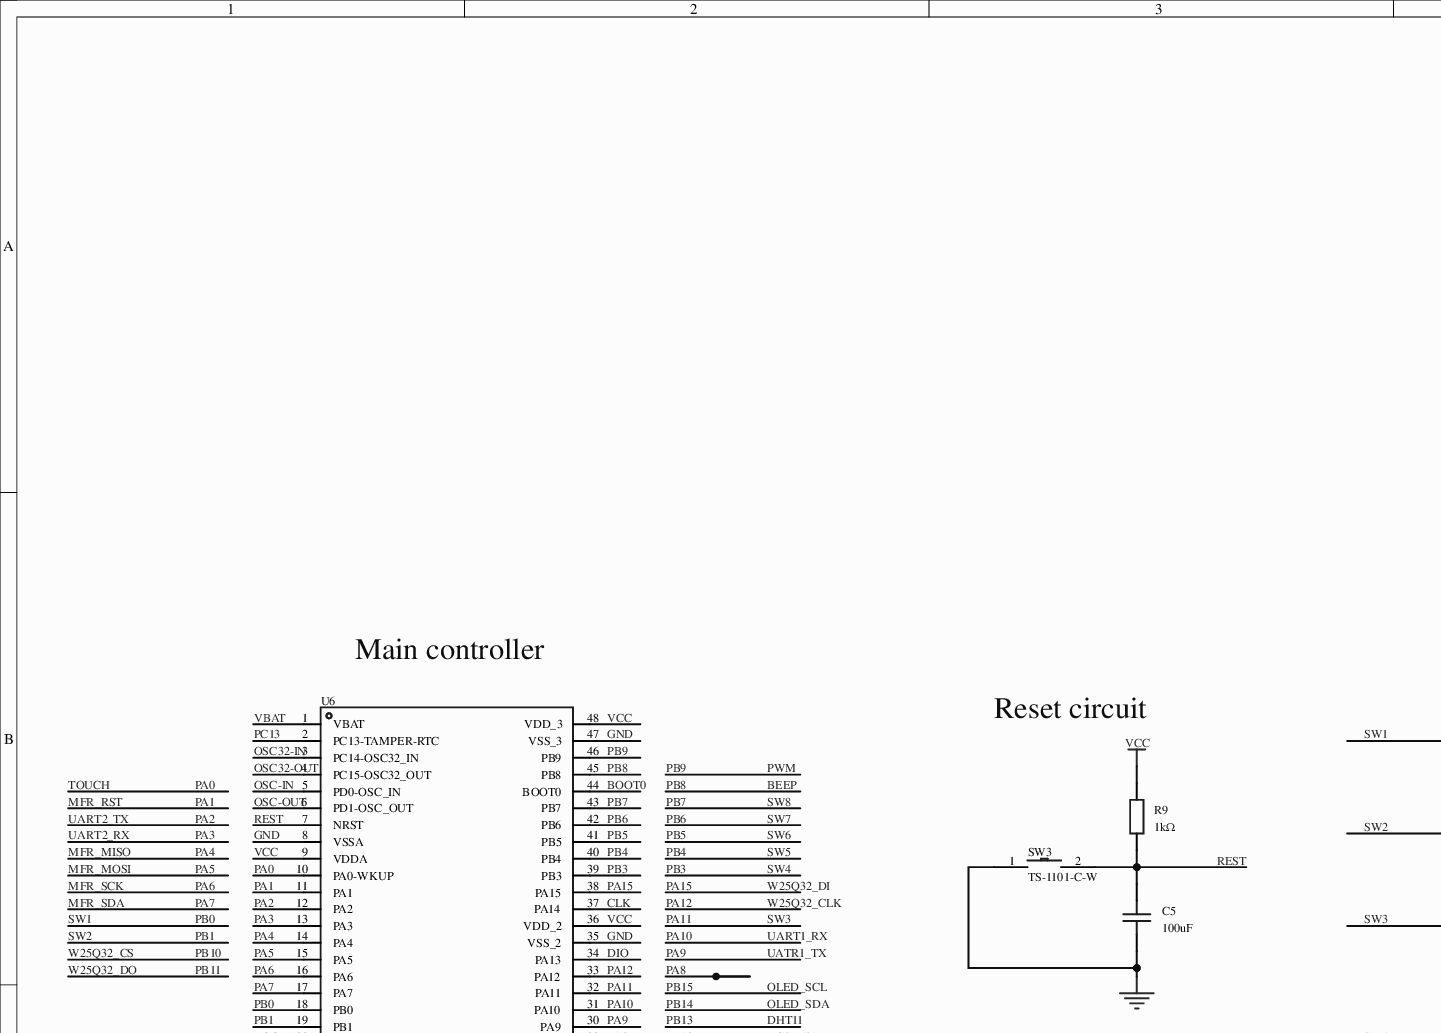
[diagram p0: MISC51820-3.schdoc, top left]
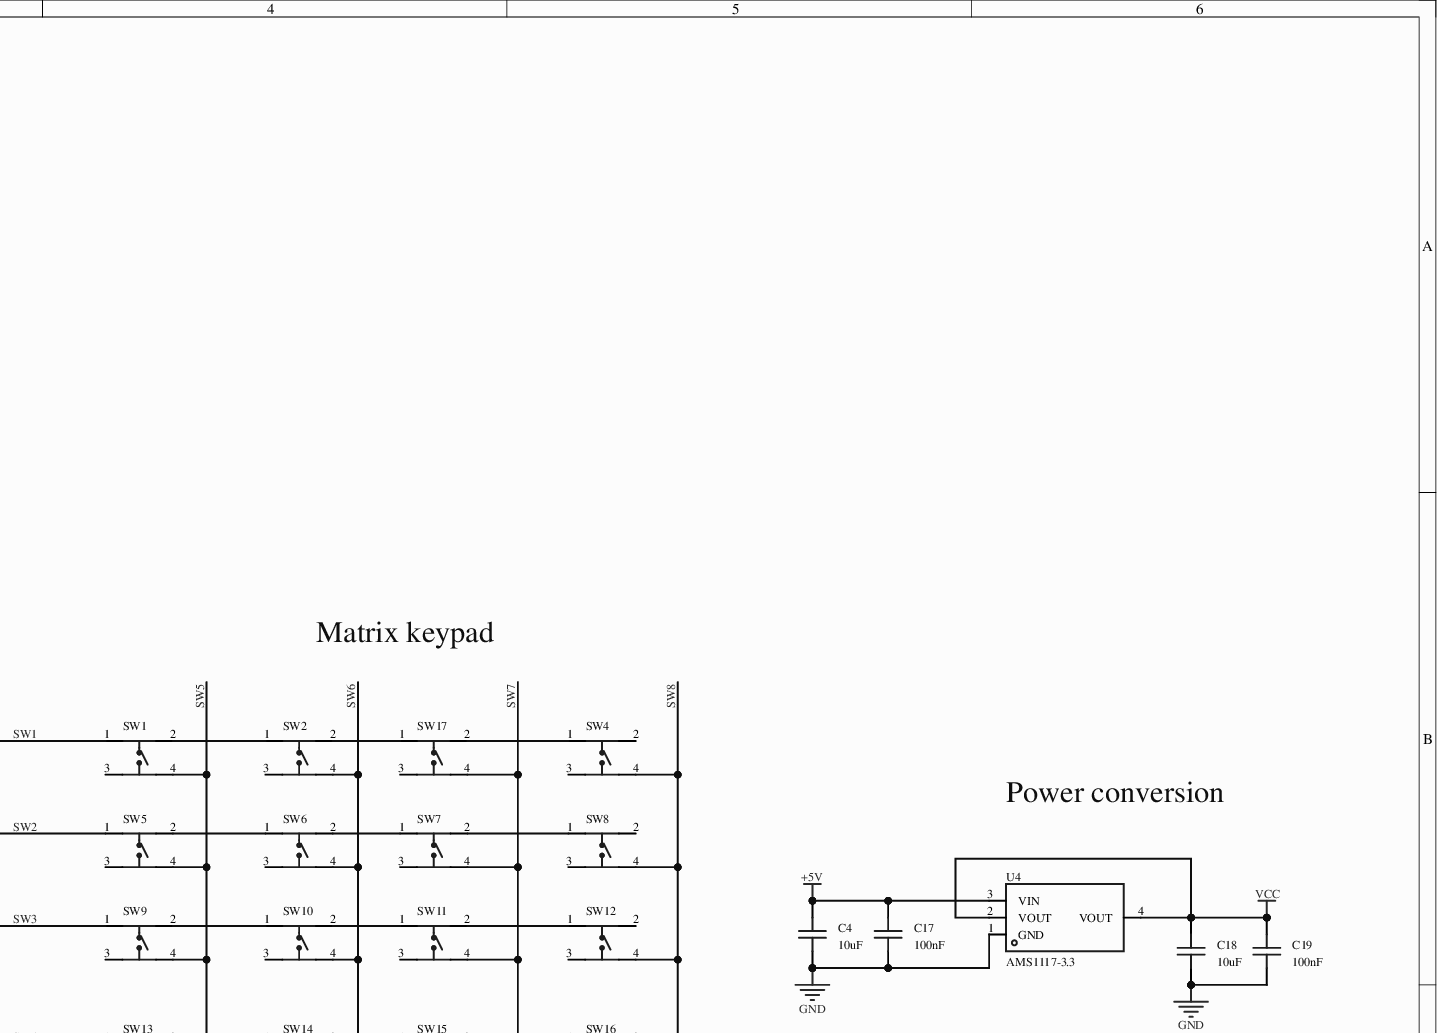
[diagram p1: MISC51820-3.schdoc, top right]
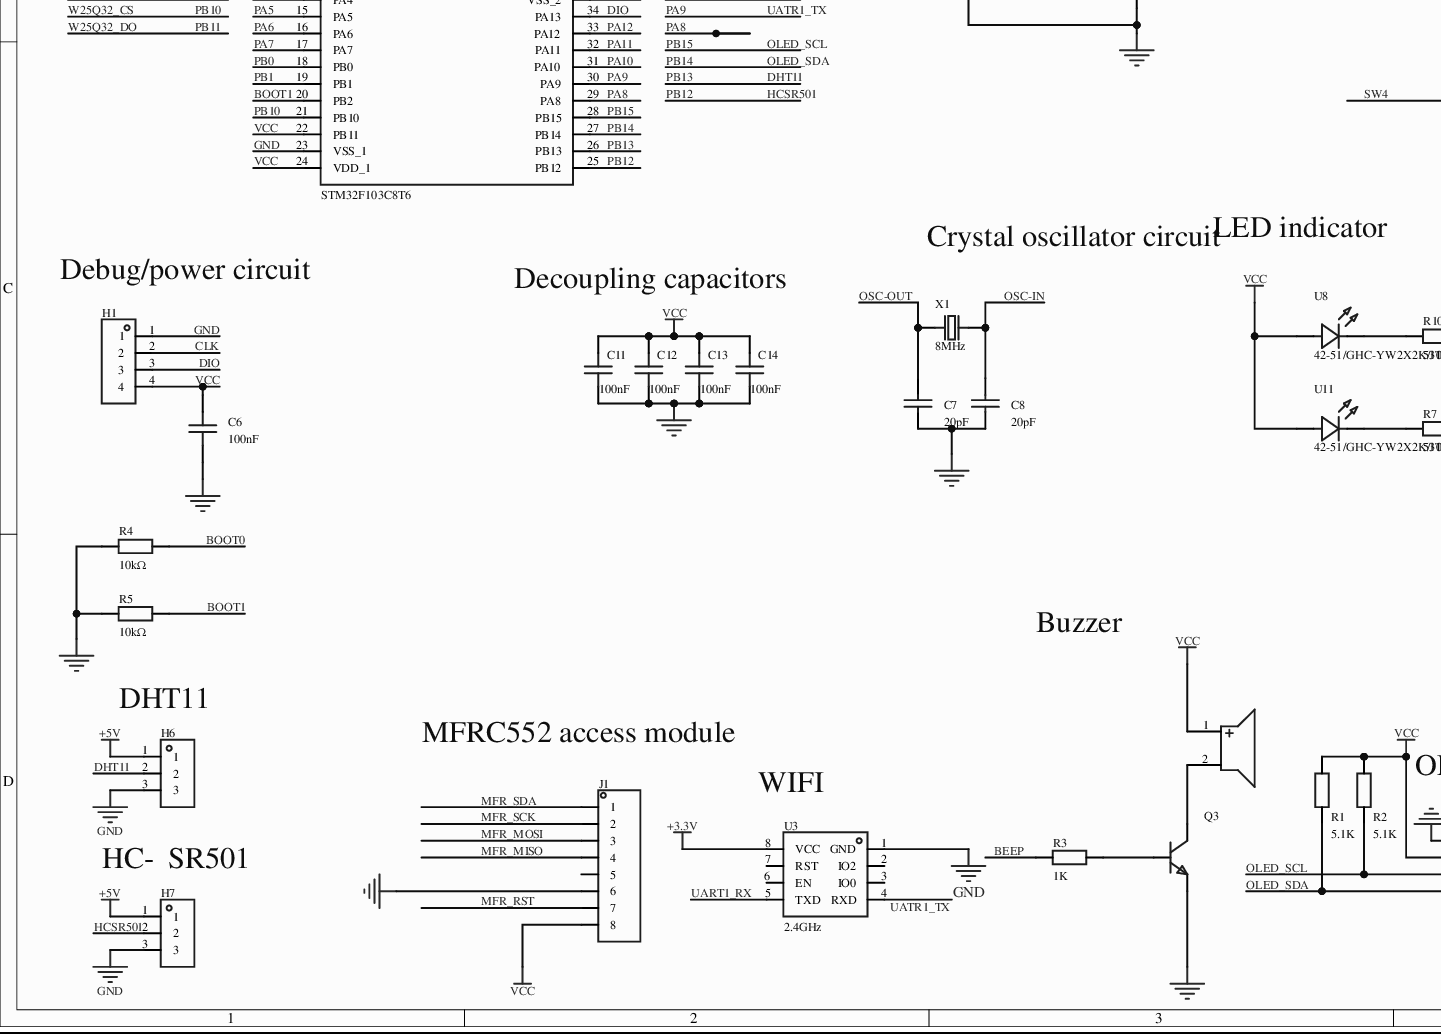
[diagram p2: MISC51820-3.schdoc, bottom left]
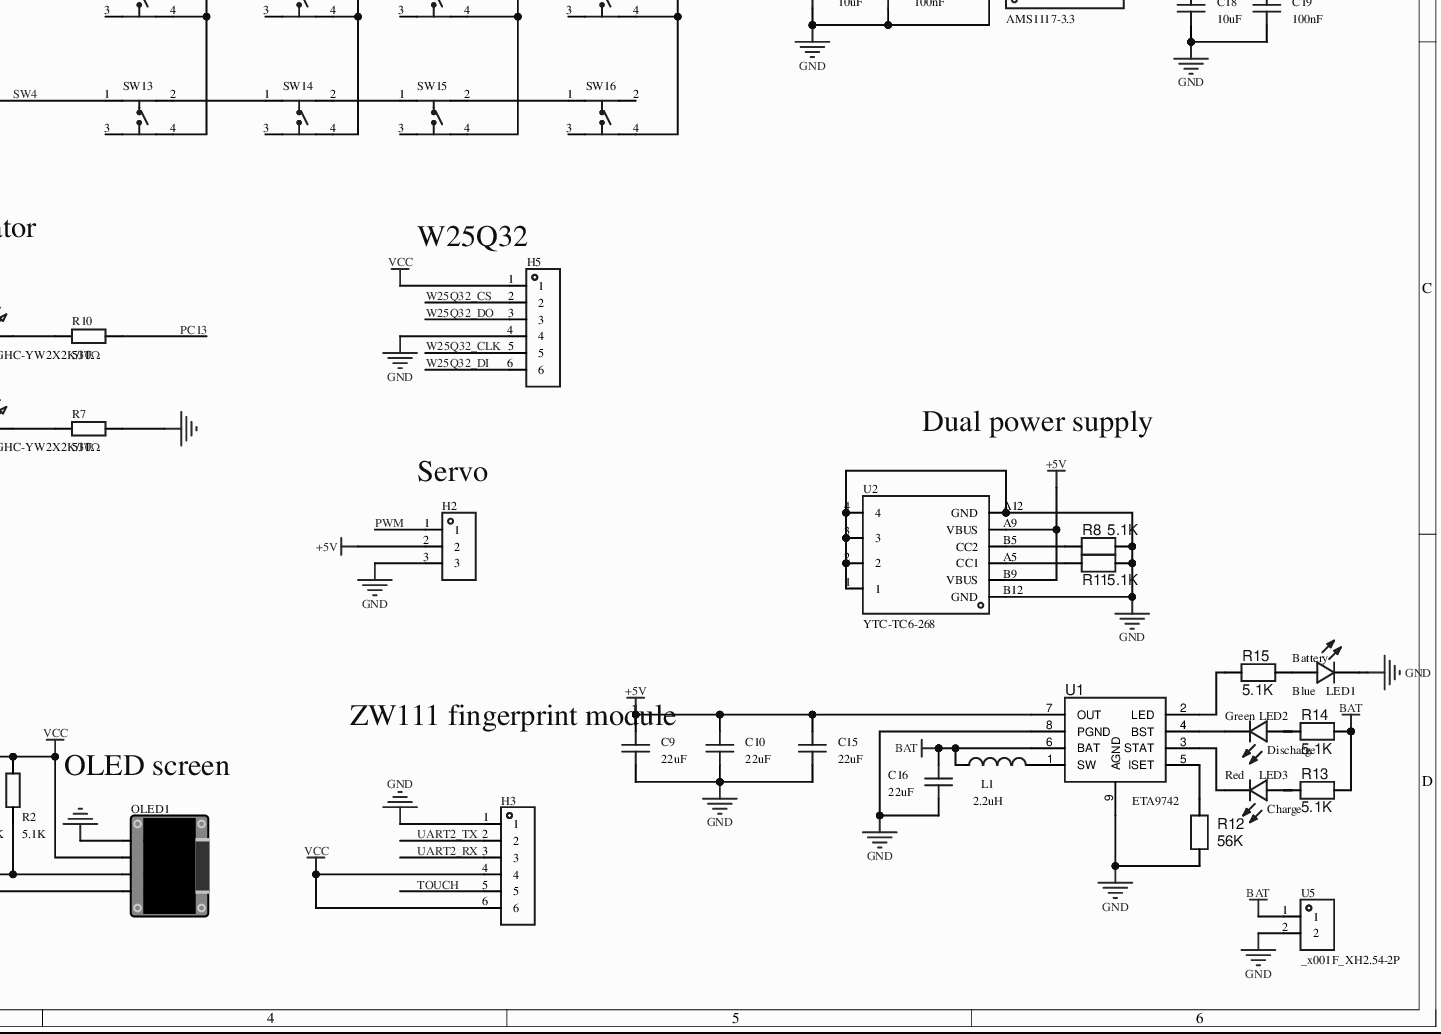
[diagram p3: MISC51820-3.schdoc, bottom right]
# Altium project MISC51820-2.PrjPcb
1 sheet, 70 parts. Net scope: global (net labels, ports and power ports of the same name join across sheets).
Board file: MISC51820.pcbdoc

## Sheet MISC51820-3.schdoc
size 420 x 297 mm; Version: V1.0; @Project Name: MISC51820; @Page Count: 1; @Update Date: 2026-04-11; @Create Date: 2026-04-11; @Schematic Name: MISC51820; @Page No: 1; @Create Time: 19:02:24; @Update Time: 19:02:29; @Board Name: MISC51820

### Parts
BUZZER1  2.7kHz  [BUZ-TH_BD9.0-P4.00-D0.6-FD]  (value not drawn)
C4  10uF  [C0603]
C5  100uF  [C1206]
C6  100nF  [C0603]
C7  20pF  [C0603]
C8  20pF  [C0603]
C9  22uF  [C0603]
C10  22uF  [C0603]
C11  100nF  [C0603]
C12  100nF  [C0603]
C13  100nF  [C0603]
C14  100nF  [C0603]
C15  22uF  [C0603]
C16  22uF  [C0603]
C17  100nF  [C0603]
C18  10uF  [C0603]
C19  100nF  [C0603]
H1  (no value)  [HDR-TH_4P-P2.54-V-F]
H2  (no value)  [HDR-TH_3P-P2.54-V-F]
H3  (no value)  [HDR-TH_6P-P2.54-V-F]
H5  (no value)  [HDR-TH_6P-P2.54-V-F]
H6  (no value)  [HDR-TH_3P-P2.54-V-F]
H7  (no value)  [HDR-TH_3P-P2.54-V-F]
J1  (no value)  [HDR-TH_8P-P2.54-V-M]
L1  2.2uH  [IND-SMD_L4.4-W4.2]
LED1  Battery  Emitted Color: Blue  [LED0603_L1.6-W0.8-RD_BLUE]
LED2  Discharge  Emitted Color: Green  [LED0603_L1.6-W0.8-RD_BLUE]
LED3  Charge  Emitted Color: Red  [LED0603_L1.6-W0.8-RD_BLUE]
OLED1  (no value)  [0.96OLED_4P]
Q3  (no value)  [S8050_TO_92]
R1  5.1K  [R0603]
R2  5.1K  [R0603]
R3  1K  [R0603]
R4  10kΩ  [R0603]
R5  10kΩ  [R0603]
R7  510Ω  [R0603]
R8  5.1K  [R0603-NSK]
R9  1kΩ  [R0603]
R10  510Ω  [R0603]
R11  5.1K  [R0603-NSK]
R12  56K  [R0603-NSK]
R13  5.1K  [R0603-NSK]
R14  5.1K  [R0603-NSK]
R15  5.1K  [R0603-NSK]
SW1  KH-6X6X6H-TJ  [SW-TH_4P-L6.0-W6.0-P4.50-LS6.5]  (value not drawn)
SW2  KH-6X6X6H-TJ  [SW-TH_4P-L6.0-W6.0-P4.50-LS6.5]  (value not drawn)
SW3  TS-1101-C-W  [SW-SMD_L6.0-W3.3-LS8.0]
SW4  KH-6X6X6H-TJ  [SW-TH_4P-L6.0-W6.0-P4.50-LS6.5]  (value not drawn)
SW5  KH-6X6X6H-TJ  [SW-TH_4P-L6.0-W6.0-P4.50-LS6.5]  (value not drawn)
SW6  KH-6X6X6H-TJ  [SW-TH_4P-L6.0-W6.0-P4.50-LS6.5]  (value not drawn)
SW7  KH-6X6X6H-TJ  [SW-TH_4P-L6.0-W6.0-P4.50-LS6.5]  (value not drawn)
SW8  KH-6X6X6H-TJ  [SW-TH_4P-L6.0-W6.0-P4.50-LS6.5]  (value not drawn)
SW9  KH-6X6X6H-TJ  [SW-TH_4P-L6.0-W6.0-P4.50-LS6.5]  (value not drawn)
SW10  KH-6X6X6H-TJ  [SW-TH_4P-L6.0-W6.0-P4.50-LS6.5]  (value not drawn)
SW11  KH-6X6X6H-TJ  [SW-TH_4P-L6.0-W6.0-P4.50-LS6.5]  (value not drawn)
SW12  KH-6X6X6H-TJ  [SW-TH_4P-L6.0-W6.0-P4.50-LS6.5]  (value not drawn)
SW13  KH-6X6X6H-TJ  [SW-TH_4P-L6.0-W6.0-P4.50-LS6.5]  (value not drawn)
SW14  KH-6X6X6H-TJ  [SW-TH_4P-L6.0-W6.0-P4.50-LS6.5]  (value not drawn)
SW15  KH-6X6X6H-TJ  [SW-TH_4P-L6.0-W6.0-P4.50-LS6.5]  (value not drawn)
SW16  KH-6X6X6H-TJ  [SW-TH_4P-L6.0-W6.0-P4.50-LS6.5]  (value not drawn)
SW17  KH-6X6X6H-TJ  [SW-TH_4P-L6.0-W6.0-P4.50-LS6.5]  (value not drawn)
U1  ETA9742  [ESOP-8_L4.9-W3.9-P1.27-LS6.0-BL-EP]
U2  YTC-TC6-268  [TYPE-C-SMD_YIYUAN_YTC-TC6-268]
U3  2.4GHz  [WIFIM-TH_8P-L24.7-W14.4-P2.54]
U4  AMS1117-3.3  [SOT-223-3_L6.5-W3.4-P2.30-LS7.0-BR]
U5  _x001F_XH2.54-2P  [CONN-TH_2P-P2.54-V]
U6  STM32F103C8T6  [LQFP-48_L7.0-W7.0-P0.50-LS9.0-BL]
U8  42-51/GHC-YW2X2K/3T  [LED-SMD_L1.6-W0.8-FD_GREEN-1]
U11  42-51/GHC-YW2X2K/3T  [LED-SMD_L1.6-W0.8-FD_GREEN-1]
X1  8MHz  [CRYSTAL-SMD_L3.2-W2.5_3225-8MHZ]

### Nets
+3.3V: U3.8(VCC)
+5V: C4.2 C9.2 C10.2 C15.2 C17.2 H2.2 H6.1 H7.1 U1.7(OUT) U2.A9(VBUS) U2.B9(VBUS) U4.3(VIN)
BAT: C16.2 L1.1 R13.1 R14.1 U1.6(BAT) U5.1
GND: C4.1 C5.1 C6.1 C7.1 C8.1 C9.1 C10.1 C11.1 C12.1 C13.1 C14.1 C15.1 C16.1 C17.1 C18.1 C19.1 H1.1 H2.3 H3.1 H5.4 H6.3 H7.3 J1.6 LED1.1(K) OLED1.1(GND) Q3.1(E) R4.1 R5.1 R7.2 R8.1 R11.1 R12.2 SW3.1 U1.8(PGND) U1.9(AGND) U2.1 U2.2 U2.3 U2.4 U2.A12(GND) U2.B12(GND) U3.1(GND) U4.1(GND) U5.2 U6.8(VSSA) U6.23(VSS_1) U6.35(VSS_2) U6.47(VSS_3)
VCC: BUZZER1.1 C6.2 C11.2 C12.2 C13.2 C14.2 C18.2 C19.2 H1.4 H3.4 H3.6 H5.1 J1.8 OLED1.2(VCC) R1.2 R2.2 R9.2 U4.2(VOUT) U4.4(VOUT) U6.9(VDDA) U6.22(PB11) U6.24(VDD_1) U6.36(VDD_2) U6.48(VDD_3) U8.1(A) U11.1(A)
BEEP: R3.2 U6.45(PB8)  [also labelled PB8]
BOOT0: R4.2 U6.44(BOOT0)
BOOT1: R5.2 U6.20(PB2)
CLK: H1.2 U6.37(PA14)
DHT11: H6.2 U6.26(PB13)  [also labelled PB13]
DIO: H1.3 U6.34(PA13)
HCSR501: H7.2 U6.25(PB12)  [also labelled PB12]
MFR_MISO: J1.4 U6.14(PA4)  [also labelled PA4]
MFR_MOSI: J1.3 U6.15(PA5)  [also labelled PA5]
MFR_RST: J1.7 U6.11(PA1)  [also labelled PA1]
MFR_SCK: J1.2 U6.16(PA6)  [also labelled PA6]
MFR_SDA: J1.1 U6.17(PA7)  [also labelled PA7]
OLED_SCL: OLED1.3(SCL) R2.1 U6.28(PB15)  [also labelled PB15]
OLED_SDA: OLED1.4(SDA) R1.1 U6.27(PB14)  [also labelled PB14]
OSC32-IN: U6.3(PC14-OSC32_IN)
OSC32-OUT: U6.4(PC15-OSC32_OUT)
OSC-IN: C8.2 U6.5(PD0-OSC_IN) X1.2
OSC-OUT: C7.2 U6.6(PD1-OSC_OUT) X1.1
PA0: H3.5 U6.10(PA0-WKUP)  [also labelled TOUCH]
PA2: H3.2 U6.12(PA2)  [also labelled UART2_TX]
PA3: H3.3 U6.13(PA3)  [also labelled UART2_RX]
PA8: U6.29(PA8)
PA9: U3.4(RXD) U6.30(PA9)  [also labelled UATR1_TX]
PA10: U3.5(TXD) U6.31(PA10)  [also labelled UART1_RX]
PA11: SW9.1 U6.32(PA11)  [also labelled SW3]
PA12: H5.5 U6.33(PA12)  [also labelled W25Q32_CLK]
PA15: H5.6 U6.38(PA15)  [also labelled W25Q32_DI]
PB0: SW1.1 U6.18(PB0)  [also labelled SW1]
PB1: SW5.1 U6.19(PB1)  [also labelled SW2]
PB3: SW13.1 U6.39(PB3)  [also labelled SW4]
PB4: SW1.4 SW5.4 SW9.4 SW13.4 U6.40(PB4)  [also labelled SW5]
PB5: SW2.4 SW6.4 SW10.4 SW14.4 U6.41(PB5)  [also labelled SW6]
PB6: SW7.4 SW11.4 SW15.4 SW17.4 U6.42(PB6)  [also labelled SW7]
PB7: SW4.4 SW8.4 SW12.4 SW16.4 U6.43(PB7)  [also labelled SW8]
PB9: H2.1 U6.46(PB9)  [also labelled PWM]
PB10: H5.2 U6.21(PB10)  [also labelled W25Q32_CS]
PB11: H5.3  [also labelled W25Q32_DO]
PC13: R10.2 U6.2(PC13-TAMPER-RTC)
REST: C5.2 R9.1 SW3.2 U6.7(NRST)
VBAT: U6.1(VBAT)
NetBUZZER1_2: BUZZER1.2 Q3.3(C)
NetL1_2: L1.2 U1.1(SW)
NetLED1_2: LED1.2(A) R15.1
NetLED2_1: LED2.1(K) U1.4(BST)
NetLED2_2: LED2.2(A) R14.2
NetLED3_1: LED3.1(K) U1.3(STAT)
NetLED3_2: LED3.2(A) R13.2
NetQ3_2: Q3.2(B) R3.1
NetR7_1: R7.1 U11.2(C)
NetR8_2: R8.2 U2.B5(CC2)
NetR10_1: R10.1 U8.2(C)
NetR11_2: R11.2 U2.A5(CC1)
NetR12_1: R12.1 U1.5(ISET)
NetR15_2: R15.2 U1.2(LED)
NetSW1_2: SW1.2 SW2.1
NetSW2_2: SW2.2 SW17.1
NetSW4_1: SW4.1 SW17.2
NetSW5_2: SW5.2 SW6.1
NetSW6_2: SW6.2 SW7.1
NetSW7_2: SW7.2 SW8.1
NetSW9_2: SW9.2 SW10.1
NetSW10_2: SW10.2 SW11.1
NetSW11_2: SW11.2 SW12.1
NetSW13_2: SW13.2 SW14.1
NetSW14_2: SW14.2 SW15.1
NetSW15_2: SW15.2 SW16.1

Not connected (* = marked no-connect by the designer): J1 5; SW1 3*; SW2 3*; SW4 2* 3*; SW5 3*; SW6 3*; SW7 3*; SW8 2* 3*; SW9 3*; SW10 3*; SW11 3*; SW12 2* 3*; SW13 3*; SW14 3*; SW15 3*; SW16 2* 3*; SW17 3*; U3 2(IO2) 3(IO0) 6(EN) 7(RST)

### Notes on the sheet
- (near U6) Main controller
- Matrix keypad
- Reset circuit
- Power conversion
- (near H1) Debug/power circuit
- Decoupling capacitors
- Crystal oscillator circuit
- LED indicator
- (near H5) W25Q32
- Dual power supply
- (near H2) Servo
- Buzzer
- DHT11
- (near C9) ZW111 fingerprint module
- (near J1) MFRC552 access module
- (near U3) WIFI
- OLED screen
- HC‑SR501

### Library data of the parts
BUZZER1 = QMB-09B-03: Drive: passive (external drive); construction: electromagnetic; frequency: 2.7kHz; sound pressure (SPL): 85dB;; Manufacturer: 华能; AddInBom: yes; ModelId: 949096c5110a440bbcfd89e7e6948986; ModelName: BUZ-TH_D9.0-H5.5-P4.0; ModelTransform: 354.33,354.33,0,90,0,0,0,0,-177.165; Voltage - Supply: 2V~5V; Symbol: QMB-09B-03; Device: QMB-09B-03; LCSC Part Name: 无源蜂鸣器QMB-09B-03; SupplierPart: C96256; ManufacturerPart: QMB-09B-03; Supplier Footprint: 插件,D=9mm; JLCPCB Part Class: Extended library; Datasheet: https://atta.szlcsc.com/upload/public/pdf/source/20210401/C96256_958B17753B5AD7CBFBCFFC7C095B4484.pdf; Supplier: LCSC; ConvertToPcb: yes; FootprintName: BUZ-TH_BD9.0-P4.00-D0.6-FD; Driver Circuitry: Passive (external drive); Technology: Electromagnetic; Value: 2.7kHz; Sound Pressure Level(SPL): 85dB; Diameter(φD): 9mm; Height: 5.7mm
C4 C17-C19 = CAP_0603: Symbol: Capacitance; 3D Model: ac125912035d415993ca9572d50418b10819f05c4eef4c71ace90d822a990e87; 3D Model Transform: 62.992,31.496,0,0,0,0,0,0,0; ConvertToPcb: yes; ModelName: C0603_L1.6-W0.8-H0.8; Device: CAP_0603; Supplier Footprint: 0603; AddInBom: yes; FootprintName: C0603
  C4 C18: Value: 10uF
  C17 C19: Value: 100nF
C5 = HGC1206R5107M100NSPJ: Capacitance: 100uF; tolerance: ±20%; rated voltage: 10V; dielectric (temperature coefficient): X5R;; Manufacturer: Chinocera(华瓷); 3D Model: e4be705b945545a48e666415e3682bd8; 3D Model Transform: 125.984,62.992,0,0,0,0,0,0,0; AddInBom: yes; ModelName: C1206_L3.2-W1.6-H1.3; Symbol: HGC1206R5107M100NSPJ; Device: HGC1206R5107M100NSPJ; LCSC Part Name: 100uF ±20% 10V; Supplier Part: C7432784; Manufacturer Part: HGC1206R5107M100NSPJ; Supplier Footprint: 1206; JLCPCB Part Class: Extended library; Datasheet: https://atta.szlcsc.com/upload/public/pdf/source/20240320/FAC3FEC40A78BC5CCCE96C232A94D860.pdf; Supplier: LCSC; Value: 100uF; Tolerance: ±20%; Voltage Rated: 10V; Temperature Coefficient: X5R; ConvertToPcb: yes; FootprintName: C1206
C6 C11-C14 = CGA0603X7R104K500JT: Capacitance: 100nF; tolerance: ±10%; rated voltage: 50V; dielectric (temperature coefficient): X7R;; Manufacturer: HRE(芯声); 3D Model: ac125912035d415993ca9572d50418b1; 3D Model Transform: 62.992,31.496,0,0,0,0,0,0,0; AddInBom: yes; ModelName: C0603_L1.6-W0.8-H0.8; Symbol: CGA0603X7R104K500JT; Device: CGA0603X7R104K500JT; LCSC Part Name: 100nF ±10% 50V; Supplier Part: C6119867; Manufacturer Part: CGA0603X7R104K500JT; Supplier Footprint: 0603; JLCPCB Part Class: Extended library; Supplier: LCSC; Value: 100nF; Tolerance: ±10%; Voltage Rated: 50V; Temperature Coefficient: X7R; ConvertToPcb: yes; FootprintName: C0603
C7 C8 = CL10C200JB8NNNC: Capacitance: 20pF; tolerance: ±5%; rated voltage: 50V; dielectric (temperature coefficient): C0G;; Manufacturer: SAMSUNG(三星); 3D Model: ac125912035d415993ca9572d50418b1; 3D Model Transform: 62.992,31.496,0,0,0,0,0,0,0; AddInBom: yes; ModelName: C0603_L1.6-W0.8-H0.8; Symbol: CL10C200JB8NNNC; Device: CL10C200JB8NNNC; LCSC Part Name: 20pF ±5% 50V; Supplier Part: C1648; Manufacturer Part: CL10C200JB8NNNC; Supplier Footprint: 0603; JLCPCB Part Class: Basic library; Datasheet: https://atta.szlcsc.com/upload/public/pdf/source/20160218/1457707763339.pdf; Supplier: LCSC; Value: 20pF; Tolerance: ±5%; Voltage Rated: 50V; Temperature Coefficient: C0G; ConvertToPcb: yes; FootprintName: C0603
C9 C10 C15 C16 = C3216X5R1V226MTJ00E: Capacitance: 22uF; tolerance: ±20%; rated voltage: 35V; dielectric (temperature coefficient): X5R;; Manufacturer: TDK; 3D Model: e4be705b945545a48e666415e3682bd8; 3D Model Transform: 125.984,62.992,0,0,0,0,0,0,0; AddInBom: yes; ModelName: C1206_L3.2-W1.6-H1.3; Symbol: C3216X5R1V226MTJ00E; Device: C3216X5R1V226MTJ00E; LCSC Part Name: 22uF ±20% 35V; Supplier Part: C342620; Manufacturer Part: C3216X5R1V226MTJ00E; Supplier Footprint: 1206; JLCPCB Part Class: Extended Part; Datasheet: https://atta.szlcsc.com/upload/public/pdf/source/20190225/C342620_AEDAF1591EBCA53DD875EA2BBF91AE9A.pdf; Supplier: LCSC; Value: 22uF; Tolerance: ±20%; Voltage Rated: 35V; Temperature Coefficient: X5R; ConvertToPcb: yes; FootprintName: C0603
H1 = HDR-F_2.54_1x4P: Symbol: 2.54-1*4P female; 3D Model: d187812051054f85879fcaa51a310d8e; 3D Model Transform: 419.6842,98.464,0,0,0,0,0,0,-118.11; ConvertToPcb: yes; Device: HDR-F_2.54_1x4P; Supplier Part: C2718488; Supplier Footprint: 插件; AddInBom: yes; FootprintName: HDR-TH_4P-P2.54-V-F; ModelName: HDR-TH_4P-P2.54-V-F
H2 = HDR-F_2.54_1x3P: Symbol: PM254V-11-03-H85; ConvertToPcb: yes; ModelId: f3b3cc5aae9641bf9e56fc160cef875b0819f05c4eef4c71ace90d822a990e87; ModelName: HDR2.54-F-LI-1X3P; ModelTransform: 299.9994,100,0,0,0,0,0,0,-118.11; Device: HDR-F_2.54_1x3P; AddInBom: yes; SupplierPart: C541850; Supplier Footprint: 插件; FootprintName: HDR-TH_3P-P2.54-V-F
H3 H5 = HDR-F_2.54_1x6P: Symbol: Header-Female-2.54_1x6; 3D Model: 0f5bcf94dcda47d085f24cdca1696fe9; 3D Model Transform: 619.684,94.488,0,0,0,0,0,0,-125.984; ConvertToPcb: yes; Device: HDR-F_2.54_1x6P; Supplier Part: C40877; Supplier Footprint: 插件; AddInBom: yes; FootprintName: HDR-TH_6P-P2.54-V-F; ModelName: HDR-TH_6P-P2.54-V-F
H6 H7 = HDR-F_2.54_1x3P: Symbol: PM254V-11-03-H85; 3D Model: f3b3cc5aae9641bf9e56fc160cef875b0819f05c4eef4c71ace90d822a990e87; 3D Model Transform: 299.9994,100,0,0,0,0,0,0,-118.11; ConvertToPcb: yes; ModelName: HDR2.54-F-LI-1X3P; Device: HDR-F_2.54_1x3P; Supplier Part: C541850; Supplier Footprint: 插件; AddInBom: yes; FootprintName: HDR-TH_3P-P2.54-V-F
J1 = HDR-M_2.54_1x8P: Symbol: Header-Male-2.54_1x8; ConvertToPcb: yes; ModelId: f5b96e27511e49e38545e53df2320202; ModelTransform: 807.87244,98.425,0,0,0,0,0,0,-118.11; Device: HDR-M_2.54_1x8P; AddInBom: yes; SupplierPart: C124381; Supplier Footprint: 插件; FootprintName: HDR-TH_8P-P2.54-V-M; ModelName: HDR-TH_8P-P2.54-V-M
L1 = MWSA0402S-2R2MT: Inductance: 2.2uH; tolerance: ±20%; rated current: 4.5A; DC resistance (DCR): 58mΩ;; Manufacturer: Sunlord(顺络); 3D Model: e9b3d3f4fa134185b54d517730715f16; 3D Model Transform: 173.228,165.354,0,0,0,0,0,0,0; AddInBom: yes; ModelName: IND-SMD_L4.2-W4.4-H2.0; Symbol: MWSA0402S-2R2MT; Device: MWSA0402S-2R2MT; LCSC Part Name: 2.2uH ±20%; Supplier Part: C408335; Manufacturer Part: MWSA0402S-2R2MT; Supplier Footprint: SMD; JLCPCB Part Class: Extended Part; Datasheet: https://atta.szlcsc.com/upload/public/pdf/source/20190729/C408335_A7E6B668A7D3CE7F04476E0D34F3244A.pdf; Supplier: LCSC; Height: 2mm; Width: 4.4mm; Value: 2.2uH; Tolerance: ±20%; Rated Current: 4.5A; DC Resistance (DCR): 58mΩ; Length: 4.2mm; ConvertToPcb: yes; FootprintName: IND-SMD_L4.4-W4.2
LED1 = NCD0603G1: Emitted color: emerald green;; Manufacturer Part: 电池; Manufacturer: 国星光电; Symbol: FC-D1608UGK-520D10; 3D Model: 1f0d29a91be547639d425604e9b96ebb; 3D Model Transform: 63.7794,32.283,0,0,0,0,0,0,0; AddInBom: yes; ModelName: LED0603-RD; Device: NCD0603G1; LCSC Part Name: 翠绿; Supplier Part: C84267; Supplier Footprint: 0603; JLCPCB Part Class: Extended Part; Datasheet: https://atta.szlcsc.com/upload/public/pdf/source/20200820/C84267_04BA7703640BAC111D09F5EFB971FBF3.pdf; Supplier: LCSC; ConvertToPcb: yes; FootprintName: LED0603_L1.6-W0.8-RD_BLUE
LED2 = NCD0603G1: Emitted color: emerald green;; Manufacturer Part: 放电; Manufacturer: 国星光电; Symbol: FC-D1608UGK-520D10; 3D Model: 1f0d29a91be547639d425604e9b96ebb; 3D Model Transform: 63.7794,32.283,0,0,0,0,0,0,0; AddInBom: yes; ModelName: LED0603-RD; Device: NCD0603G1; LCSC Part Name: 翠绿; Supplier Part: C84267; Supplier Footprint: 0603; JLCPCB Part Class: Extended Part; Datasheet: https://atta.szlcsc.com/upload/public/pdf/source/20200820/C84267_04BA7703640BAC111D09F5EFB971FBF3.pdf; Supplier: LCSC; ConvertToPcb: yes; FootprintName: LED0603_L1.6-W0.8-RD_BLUE
LED3 = NCD0603G1: Emitted color: emerald green;; Manufacturer Part: 充电; Manufacturer: 国星光电; Symbol: FC-D1608UGK-520D10; 3D Model: 1f0d29a91be547639d425604e9b96ebb; 3D Model Transform: 63.7794,32.283,0,0,0,0,0,0,0; AddInBom: yes; ModelName: LED0603-RD; Device: NCD0603G1; LCSC Part Name: 翠绿; Supplier Part: C84267; Supplier Footprint: 0603; JLCPCB Part Class: Extended Part; Datasheet: https://atta.szlcsc.com/upload/public/pdf/source/20200820/C84267_04BA7703640BAC111D09F5EFB971FBF3.pdf; Supplier: LCSC; ConvertToPcb: yes; FootprintName: LED0603_L1.6-W0.8-RD_BLUE
OLED1 = 0.96OLED模块_4P: Symbol: 0.96OLED module_4P; ConvertToPcb: yes; ModelId: 79c000fdb68d45a296c2e9bedf4f90550819f05c4eef4c71ace90d822a990e87; ModelTransform: 1393.69792,1318.895,0,0,0,0,0,-560.079,-137.795; Device: 0.96OLED module_4P; AddInBom: yes; FootprintName: 0.96OLED_4P; Supplier Footprint: 插件; ModelName: 0.96OLED_4P
Q3 = S8050_TO_NPN: ConvertToPcb: yes; ModelId: aafe8e06f2154e7c93506efd0d6632dd; ModelName: TO-92-3_L4.9-W3.7-P1.27-L; ModelTransform: 180.78,141.44,417.3,0,0,0,0,0,-200; Device: S8050_TO_NPN; Symbol: S8050_TO_NPN; AddInBom: yes; Supplier Footprint: TO-92; FootprintName: S8050_TO_92
R1 R2 = Res_0603: Symbol: Resistor; ConvertToPcb: yes; ModelId: fc143cca1e79419f9cd78b61e9279f080819f05c4eef4c71ace90d822a990e87; ModelTransform: 31.8897,63.7794,0,90,0,0,0,0,0; Device: Res_0603; Value: 5.1K; AddInBom: yes; Supplier Footprint: 0603; FootprintName: R0603; ModelName: R0603
R3 = Res_0603: Symbol: Resistor; 3D Model: fc143cca1e79419f9cd78b61e9279f080819f05c4eef4c71ace90d822a990e87; 3D Model Transform: 31.8897,63.7794,0,90,0,0,0,0,0; ConvertToPcb: yes; Device: Res_0603; Value: 1K; Supplier Footprint: 0603; AddInBom: yes; FootprintName: R0603; ModelName: R0603
R4 R5 = 0603WAF1002T5E: Resistor type: thick film resistor; resistance: 10kΩ; tolerance: ±1%; power: 100mW; max working voltage: 75V; temperature coefficient: ±100ppm/℃;; Manufacturer: UNI-ROYAL(厚声); 3D Model: fc143cca1e79419f9cd78b61e9279f08; 3D Model Transform: 31.8897,63.7794,0,90,0,0,0,0,0; AddInBom: yes; Symbol: 0603WAF1002T5E; Device: 0603WAF1002T5E; LCSC Part Name: 厚膜电阻 10kΩ ±1% 100mW; Supplier Part: C25804; Manufacturer Part: 0603WAF1002T5E; Supplier Footprint: 0603; JLCPCB Part Class: Basic library; Datasheet: https://atta.szlcsc.com/upload/public/pdf/source/20200306/C422600_1E6D84923E4A46A82E41ADD87F860B5C.pdf; Supplier: LCSC; Type: Thick film resistor; Value: 10kΩ; Tolerance: ±1%; Power(Watts): 100mW; Overload Voltage (Max): 75V; Temperature Coefficient: ±100ppm/℃; Operating Temperature Range: -55℃~+155℃; ConvertToPcb: yes; FootprintName: R0603; ModelName: R0603
R7 R10 = 0603WAF5100T5E: Resistor type: thick film resistor; resistance: 510Ω; tolerance: ±1%; power: 100mW; max working voltage: 75V; temperature coefficient: ±100ppm/℃;; Manufacturer: UNI-ROYAL(厚声); 3D Model: fc143cca1e79419f9cd78b61e9279f08; 3D Model Transform: 31.8897,63.7794,0,90,0,0,0,0,0; AddInBom: yes; Symbol: 0603WAF5100T5E; Device: 0603WAF5100T5E; LCSC Part Name: 510Ω ±1% 100mW 厚膜电阻; Supplier Part: C23193; Manufacturer Part: 0603WAF5100T5E; Supplier Footprint: 0603; JLCPCB Part Class: Basic library; Datasheet: https://atta.szlcsc.com/upload/public/pdf/source/20200306/C422600_1E6D84923E4A46A82E41ADD87F860B5C.pdf; Supplier: LCSC; Type: Thick film resistor; Value: 510Ω; Tolerance: ±1%; Power(Watts): 100mW; Overload Voltage (Max): 75V; Temperature Coefficient: ±100ppm/℃; Operating Temperature Range: -55℃~+155℃; ConvertToPcb: yes; FootprintName: R0603; ModelName: R0603
R8 R11-R15 = NC: Add into BOM: yes; Symbol: NC; Device: NC; Convert to PCB: yes; Origin Footprint: R0603-NSK; FootprintName: R0603-NSK
R9 = RC0603FR-071KL: Resistor type: thick film resistor; resistance: 1kΩ; tolerance: ±1%; power: 100mW; max working voltage: 75V; temperature coefficient: ±100ppm/℃;; Manufacturer: YAGEO(国巨); 3D Model: fc143cca1e79419f9cd78b61e9279f08; 3D Model Transform: 31.8897,63.7794,0,90,0,0,0,0,0; AddInBom: yes; Symbol: RC0603FR-071KL; Device: RC0603FR-071KL; LCSC Part Name: 厚膜电阻 1kΩ ±1% 100mW; Supplier Part: C22548; Manufacturer Part: RC0603FR-071KL; Supplier Footprint: 0603; JLCPCB Part Class: Extended library; Datasheet: https://atta.szlcsc.com/upload/public/pdf/source/20180316/70C0E2BDAE7FCC62C531A5A58D202EE1.pdf; Supplier: LCSC; Type: Thick film resistor; Value: 1kΩ; Tolerance: ±1%; Power(Watts): 100mW; Overload Voltage (Max): 75V; Temperature Coefficient: ±100ppm/℃; Operating Temperature Range: -55℃~+155℃; ConvertToPcb: yes; FootprintName: R0603; ModelName: R0603
SW1 SW2 SW4-SW17 = KH-6X6X6H-TJ: 电路结构:单刀单掷;按钮形状:圆形按钮;作用力:2.6N;安装方式:直插;开关长度:6mm;开关宽度:6mm;开关高度:6mm;带支架:不带支架;触点电流:50mA;额定电压:12V;工作寿命:-;; Manufacturer: kinghelm(金航标); 3D Model: 20eee248bc684ccd8cbdbb1d0d91ec6f; 3D Model Transform: 236.22,323.03,0,90,0,0,0,0,-137.795; Circuit: SPST; Actuator Style: Round button; Operating Force: 2.6N; Switch Height: 6mm; with Bracket: Without bracket; Contact Current: 50mA; Voltage Rating: 12V; Actuator/Cap Color: Black; AddInBom: yes; ModelName: SW-TH_4P-L6.0-W6.0-H5.0-LS6.5-P4.50; Symbol: KH-6X6X6H-TJ; Device: KH-6X6X6H-TJ; LCSC Part Name: 6*6*6mm 直插 轻触开关; Supplier Part: C2837516; Manufacturer Part: KH-6X6X6H-TJ; Supplier Footprint: 插件-4P,6x6mm; JLCPCB Part Class: Extended library; Datasheet: https://item.szlcsc.com/datasheet/KH-6X6X6H-TJ/3009586.html; Supplier: LCSC; Mounting Type: Through-hole; Length: 6mm; Width: 6mm; Termination Style: PC pins; Life: -; Operating Temperature: -25℃~+70℃; ConvertToPcb: yes; FootprintName: SW-TH_4P-L6.0-W6.0-P4.50-LS6.5
SW3 = TS-1101-C-W: 电路结构:单刀单掷;按钮形状:矩形按钮;作用力:260gf;安装方式:立贴;开关长度:6mm;开关宽度:3.6mm;开关高度:2.5mm;带支架:不带;触点电流:50mA;额定电压(AC):-;额定电压(DC):12V;额定功率:-;绝缘电阻:-;带灯:无;机械寿命:5万次;; Manufacturer: XKB Connectivity(中国星坤); 3D Model: b2f4ea9f0afc4b0786d53dba66ceb9e4; 3D Model Transform: 314.96,129.921,0,0,0,0,0,0,0; Circuit: SPST; Actuator Style: Rectangular button; Operating Force: 260gf; Switch Length: 6mm; Switch Width: 3.6mm; Switch Height: 2.5mm; Strike Gundam: Without; Contact Current: 50mA; Voltage Rating (DC): 12V; Actuator/Cap Color: White, light green tint; With Lamp: None; Mechanical Life: 5万 cycles; AddInBom: yes; ModelName: SW-SMD_L6.0-W3.3-H5-LS8.0; Symbol: TS-1101-C-W; Device: TS-1101-C-W; LCSC Part Name: 6*3.6*2.5mm 立贴 轻触开关; Supplier Part: C318938; Manufacturer Part: TS-1101-C-W; Supplier Footprint: SMD; JLCPCB Part Class: Extended library; Datasheet: https://atta.szlcsc.com/upload/public/pdf/source/20200227/C318938_C2E53B1EEDE37D980A33616AC086DE53.pdf; Supplier: LCSC; Mounting Style: Surface mount; Voltage Rating (AC): -; Power Rating: -; Insulation Resistance: -; IP Rating: -; Pin Style: -; Operating Temperature: -30℃~+85℃; ConvertToPcb: yes; FootprintName: SW-SMD_L6.0-W3.3-LS8.0
U1 = ETA9742: Manufacturer: 钰泰; AddInBom: yes; Symbol: ETA9742; Device: ETA9742; Supplier: 钰泰; Origin Footprint: ESOP-8_L4.9-W3.9-P1.27-LS6.0-BL-EP; ConvertToPcb: yes; FootprintName: ESOP-8_L4.9-W3.9-P1.27-LS6.0-BL-EP
U2 = YTC-TC6-268: Connector type: Type-C; gender: female socket; contacts: 6;; Manufacturer: YIYUAN(怡远); 3D Model: 1d7009b8f1724e38b5608beb74744d7c; 3D Model Transform: 351.9678,271.653,0,0,0,0,0,-49.21,-39.37; Number of Contacts: 6; AddInBom: yes; Symbol: YTC-TC6-268; Device: YTC-TC6-268; LCSC Part Name: Type-C 母座; Supplier Part: C5260484; Manufacturer Part: YTC-TC6-268; Supplier Footprint: SMD; JLCPCB Part Class: Extended Part; Datasheet: https://atta.szlcsc.com/upload/public/pdf/source/20221115/94102468E8C367463F1D717839C68408.pdf; Supplier: LCSC; Connector Type: Type-C; Gender: Female socket; ConvertToPcb: yes; FootprintName: TYPE-C-SMD_YIYUAN_YTC-TC6-268; ModelName: TYPE-C-SMD_YIYUAN_YTC-TC6-268
U3 = ESP-01S: Core processor: ESP8266 chip; frequency: 2.4GHz; antenna form: onboard PCB antenna; transmit power: 16dBm; receive sensitivity: -90dBm;; Manufacturer: Ai-Thinker(安信可); Symbol: ESP-01S_C503582; 3D Model: 9453774c1eaa4779b246df5901e962460819f05c4eef4c71ace90d822a990e87; 3D Model Transform: 972.43904,566.928,0,0,0,0,377.167,-3.936,-118.11; Support Interface: GPIO; UART; PWM; Operating Voltage: 3V~3.6V; Receive  Current: 56mA; Send  Current: 170mA; AddInBom: yes; ModelName: WIFIM-TH_8P-L24.7-W14.4-H2.8-P2.54; Device: ESP-01S; LCSC Part Name: 完整的802.11b/g/nWi-FiSoC模块; Supplier Part: C503582; Manufacturer Part: ESP-01S; Supplier Footprint: -; JLCPCB Part Class: Extended Part; Datasheet: https://atta.szlcsc.com/upload/public/pdf/source/20200407/C503582_1139AF8FB42E05635FA0089E1752A536.pdf; Supplier: LCSC; Core Processor: ESP8266 chip; Wireless Standard: -; Value: 2.4GHz; Antenna Type: Onboard PCB antenna; Output Power: 16dBm; Sensitivity: -90dBm; Operating Temperature: -20℃~+70℃; ConvertToPcb: yes; FootprintName: WIFIM-TH_8P-L24.7-W14.4-P2.54
U4 = AMS1117-3.3_C6186: Output type: fixed; working voltage: 15V; output voltage: 3.3V; output current: 1A; power supply rejection ratio (PSRR): 72dB@(120Hz); output polarity: positive;; Manufacturer: AMS; AddInBom: yes; ModelId: 925194bf9823436183a3e0b978a8d0760819f05c4eef4c71ace90d822a990e87; ModelName: SOT-223-4P_L6.5-W3.5-H1.6-LS7.0-P2.30; ModelTransform: 279.89794,255.905,0,180,0,0,-3.9385,-0.0005,0; Voltage Dropout: 1.1V@(800mA); standby current: 5mA; Noise: 0.003%Vout; Number of Outputs: 1; Symbol: AMS1117-3.3; Device: AMS1117-3.3_C6186; LCSC Part Name: 3.3V 1A 15V; SupplierPart: C6186; ManufacturerPart: AMS1117-3.3; Supplier Footprint: SOT-223; JLCPCB Part Class: Basic Part; Datasheet: https://item.szlcsc.com/datasheet/AMS1117-3.3/6652.html; Supplier: LCSC; ConvertToPcb: yes; FootprintName: SOT-223-3_L6.5-W3.4-P2.30-LS7.0-BR; Output Type: Fixed; Voltage - Supply: 15V; Output Voltage: 3.3V; Output Current: 1A; Power Supply Rejection Ratio (PSRR): 72dB@(120Hz); Features: Overcurrent protection; thermal shutdown; Operating Temperature: -40℃~+125℃; Output Configuration: Positive
U5 = _x001F_XH2.54-2P: AddInBom: yes; ModelId: 4b619f877c224111ac90f050b36c35830819f05c4eef4c71ace90d822a990e87; ModelTransform: 295.275,224.409,0,180,0,0,0,17.717,-118.11; Symbol: _X001F_XH2.54-2P; Device: _x001F_XH2.54-2P; LCSC Part Name: _x001F_XH2.54-2P; SupplierPart: C9900016027; ManufacturerPart: _x001F_XH2.54-2P; Supplier Footprint: XH2.54-2P直插; JLCPCB Part Class: Extended Part; Supplier: LCSC; ConvertToPcb: yes; FootprintName: CONN-TH_2P-P2.54-V; ModelName: CONN-TH_2P-P2.54-V
U6 = STM32F103C8T6: CPU内核:ARM-M3;程序存储容量:64KB;RAM总容量:20KB;GPIO端口数量:37;工作电压范围:2V~3.6V;CPU最大主频:72MHz;程序存储器类型:FLASH;; Manufacturer: ST(意法半导体); 3D Model: 093be70396ff421eb2cdb946d5311efc; 3D Model Transform: 354.331,354.331,0,0,0,0,0,0,0; CPU Core: ARM-M3; Program Storage Size: 64KB; RAM Size: 20KB; GPIO Ports Number: 37; CPU Maximum Speed: 72MHz; Program Memory Type: FLASH; ADC (Bit): 12bit; Universal Serial Bus: Yes; Peripheral/Function: Watchdog; DMA; watchdog; temperature sensor; ModelName: LQFP-48_L7.0-W7.0-H1.4-LS9.0-P0.50; Symbol: STM32F103C8T6; Device: STM32F103C8T6; LCSC Part Name: 主流增强型ARM Cortex-M3 MCU，具有64 KB Flash、72 MHz CPU、电机控制、USB和CAN; Supplier Part: C8734; Manufacturer Part: STM32F103C8T6; Supplier Footprint: LQFP-48(7x7); JLCPCB Part Class: Extended library; Datasheet: https://atta.szlcsc.com/upload/public/pdf/source/20220812/8363ACEC51AD55ECEB84799464F7CB85.pdf; Supplier: LCSC; Operating Voltage Range: 2V~3.6V; Operating Temperature Range: -40℃~+85℃; DAC (Bit): -; PWM (Bit): -; Internal Comparator: -; communication protocol: -; Watchdog: Yes; Real-Time Clock: -; Infrared Data Association: Yes; Low-Voltage Detect: Yes; CCP Capture/Compare: -; Secure Digital Input and Output: -; Direct Memory Access: Yes; Internal Oscillator: Yes; AddInBom: yes; ConvertToPcb: yes; FootprintName: LQFP-48_L7.0-W7.0-P0.50-LS9.0-BL
U8 U11 = 42-51/GHC-YW2X2K/3T: Emitted color: emerald green; forward current: -; dominant wavelength: 520nm~535nm; luminous intensity: 2850mcd;; Manufacturer: EVERLIGHT(亿光); 3D Model: feee2acead2344579596fed70e7e7f0f; 3D Model Transform: 63.7794,31.89954,0,0,0,0,0,0,0; AddInBom: yes; Symbol: 42-51/GHC-YW2X2K/3T; Device: 42-51/GHC-YW2X2K/3T; LCSC Part Name: 正发光贴片灯 颜色正绿色 发光二极管; Supplier Part: C5136797; Manufacturer Part: 42-51/GHC-YW2X2K/3T; Supplier Footprint: 0603; JLCPCB Part Class: Extended library; Datasheet: https://atta.szlcsc.com/upload/public/pdf/source/20220916/FBE88CF67A3FC292A254CF6ACE30EBDE.pdf; Supplier: LCSC; Emitted Color: Emerald green; Forward Current: -; Dominant Wavelength: 520nm~535nm; Luminous Intensity: 2850mcd; ConvertToPcb: yes; FootprintName: LED-SMD_L1.6-W0.8-FD_GREEN-1; ModelName: LED-SMD_L1.6-W0.8-FD_GREEN-1
X1 = X22EL89COI-111YLC-8M: Crystal type: SMD crystal; frequency: 8MHz; room-temperature frequency tolerance: ±10ppm; load capacitance: 12pF; frequency stability: ±20ppm;; Manufacturer: YXC(扬兴晶振); AddInBom: yes; ModelId: 28ce33d39be745caa449ad3e35d8096d0819f05c4eef4c71ace90d822a990e87; ModelTransform: 125.984,98.425,0,0,0,0,0,0,0; Symbol: X22EL89COI-111YLC-8M; Device: X22EL89COI-111YLC-8M; LCSC Part Name: YSX320GA 8MHZ 12PF ±10PPM -40~85℃ (±20PPM); SupplierPart: C42448903; ManufacturerPart: X22EL89COI-111YLC-8M; Supplier Footprint: SMD3225-2P; JLCPCB Part Class: Extended Part; Datasheet: https://item.szlcsc.com/datasheet/X22EL89COI-111YLC-8M/44509786.html; Supplier: LCSC; ConvertToPcb: yes; FootprintName: CRYSTAL-SMD_L3.2-W2.5_3225-8MHZ; ModelName: CRYSTAL-SMD_L3.2-W2.5_3225-8MHZ; Type: SMD crystal; Value: 8MHz; Normal temperature Frequency Tolerance: ±10ppm; Load Capacitance: 12pF; Frequency Stability: ±20ppm; Operating Temperature: -40℃~+85℃